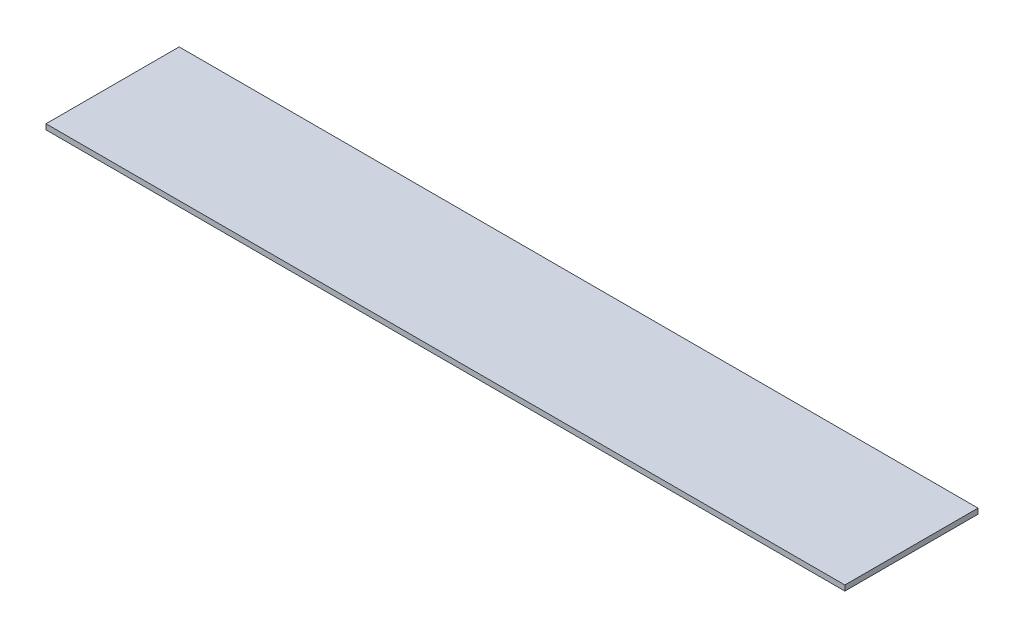
from build123d import *

# Parameters (mm, degrees)
SKETCH_1_W      = 600
SKETCH_1_H      = 100
EXTRUDE_1_DEPTH = 4


with BuildPart() as part:
    # 草图1 → 凸台-拉伸1 (new body)
    with BuildSketch(Plane(origin=(0, 0, 0), x_dir=(1, 0, 0), z_dir=(0, 1, 0))):
        with Locations((300, 50)):
            Rectangle(SKETCH_1_W, SKETCH_1_H)
    extrude(amount=EXTRUDE_1_DEPTH)


solid = part.part
